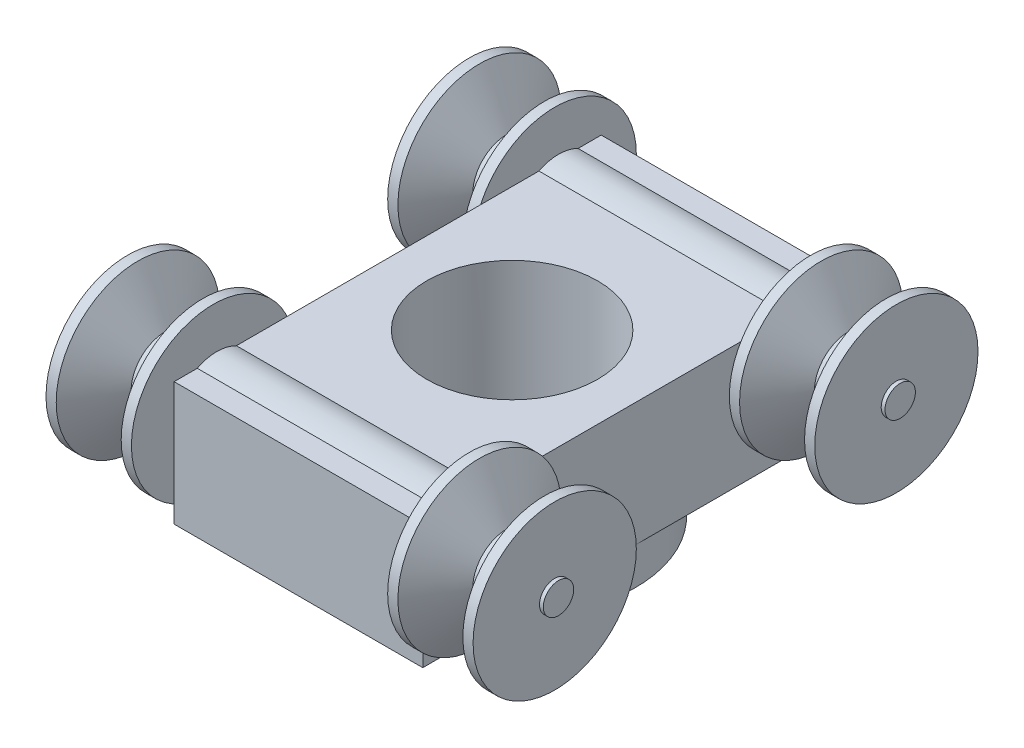
SolidWorks part; units mm, degrees
ref_plane "Front Plane" through (0, 0, 0) normal (0, 0, 1) x (1, 0, 0)
ref_plane "Top Plane" through (0, 0, 0) normal (0, 1, 0) x (1, 0, 0)
ref_plane "Right Plane" through (0, 0, 0) normal (1, 0, 0) x (0, 0, -1)
sketch "Sketch2" plane through (0, 0, 0) normal (0, 1, 0) x (1, 0, 0)
  line L0 (0, 0) -> (0, 35)
  line L2 (5.3868, 35) -> (19.8205, 10)
  line L3 (19.8205, 10) -> (25.1795, 10)
  line L4 (25.1795, 10) -> (39.6132, 35)
  line L6 (45, 35) -> (45, 0)
  line L7 (45, 0) -> (0, 0)
  line L8 (22.5, 0) -> (22.5, 10) construction
  line L9 (10.8921, -8) -> (33.1251, -8) construction
  line L10 (0, 35) -> (5.3868, 35)
  line L11 (39.6132, 35) -> (45, 35)
  dimension "D1" = 45
  dimension "D2" = 60
  dimension "D3" = 60
  dimension "D6" = 10
  dimension "D8" = 8
revolve "Revolve1" add sketch "Sketch2" angle 360 about L9
pattern_linear "LPattern1" count 2 spacing 180 along (1, 0, 0) of "Revolve1"
sketch "Sketch3" plane through (45, 0, 0) normal (1, 0, 0) x (0, 0, -1)
  circle A0 centre (-8, 0) radius 22.5
  dimension "D1" = 45
extrude "Boss-Extrude2" add sketch "Sketch3" along normal blind 135
sketch "Sketch4" plane through (45, 0, 0) normal (1, 0, 0) x (0, 0, -1)
  circle A0 centre (-8, 0) radius 30.4124
  circle A1 centre (-8, 0) radius 16
  dimension "D1" = 32
extrude "Cut-Extrude1" cut sketch "Sketch4" along normal blind 2
ref_plane "Plane4" through (112.5, 0, 0) normal (-1, 0, 0) x (0, 0, 1)
mirror "Mirror1" about plane through (112.5, 0, 0) normal (-1, 0, 0) of "Cut-Extrude1"
sketch "Sketch5" plane through (180, 0, 0) normal (1, 0, 0) x (0, 0, -1)
  circle A0 centre (-8, 0) radius 8
extrude "Boss-Extrude3" add sketch "Sketch5" along normal blind 47
mirror "Mirror2" about plane through (112.5, 0, 0) normal (-1, 0, 0) of "Boss-Extrude3"
pattern_linear "LPattern2" count 2 spacing 180 along (0, 0, 1) of bodies 108
sketch "Sketch6" plane through (0, 0, 0) normal (0, 1, 0) x (1, 0, 0)
  line L1 (47, 14.5) -> (178, 14.5)
  line L2 (47, 14.5) -> (47, -210.5)
  line L3 (47, -210.5) -> (178, -210.5)
  line L4 (178, 14.5) -> (178, -210.5)
extrude "Boss-Extrude4" add sketch "Sketch6" along normal blind 20 and the other way blind 45
sketch "Sketch7" plane through (0, -45, 0) normal (0, -1, 0) x (1, 0, 0)
  line L0 (112.5, 210.5) -> (112.5, -14.637) construction
  line L1 (47, 210.5) -> (178, 210.5) construction
  line L2 (112.5, 47.3) -> (112.5, -47.3) construction
  circle A0 centre (112.5, 97.9315) radius 65
  dimension "D1" = 130
extrude "Boss-Extrude5" add sketch "Sketch7" along normal blind 20
sketch "Sketch8" plane through (0, -65, 0) normal (0, -1, 0) x (1, 0, 0)
  circle A0 centre (112.5, 97.9315) radius 45
  dimension "D1" = 90
extrude "Cut-Extrude2" cut sketch "Sketch8" against normal through all both and the other way through all
